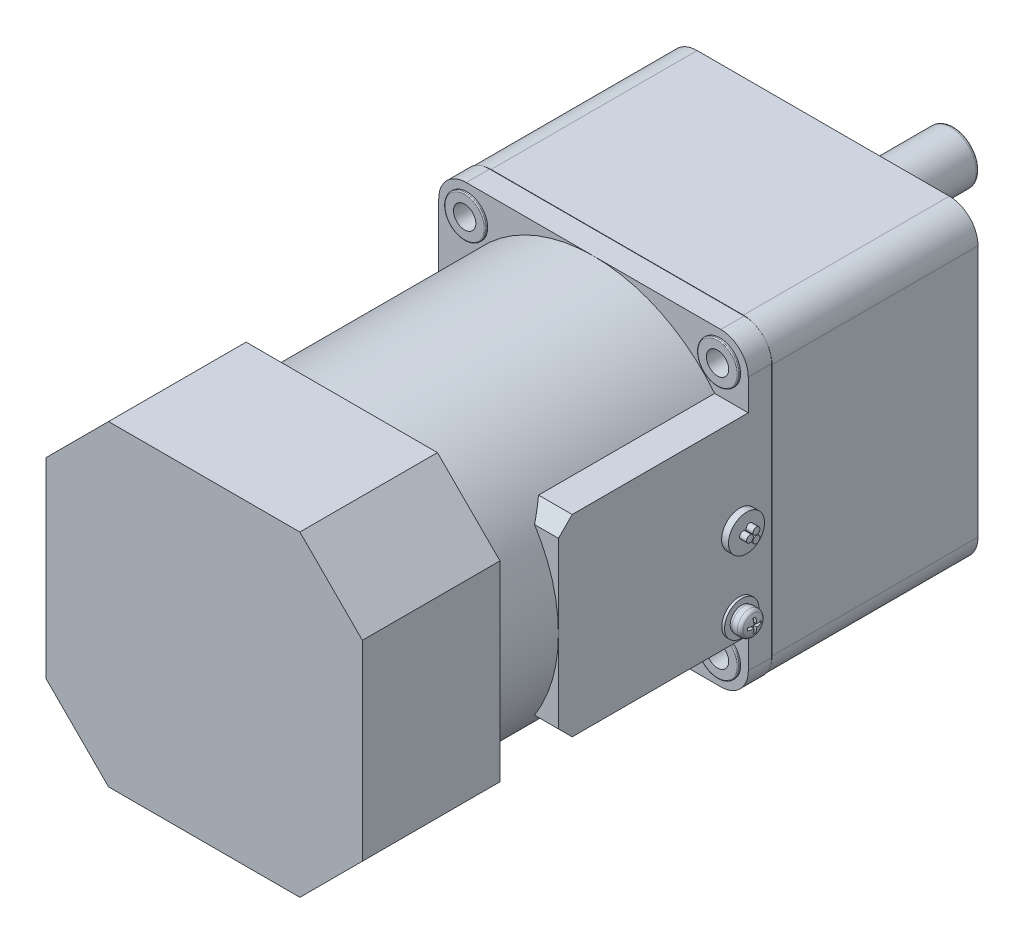
from build123d import *

# Parameters (mm, degrees)
EXTRUDE_1_DEPTH             = 60
EXTRUDE_2_DEPTH             = 6.8
SKETCH_4_W                  = 90
SKETCH_4_H                  = 90
CUT_EXTRUDE_1_DEPTH         = 0.1
EXTRUDE_3_DEPTH             = 45
PATTERN_LINEAR_1_COUNT      = 2
PATTERN_LINEAR_1_PITCH      = 73.539105243
PATTERN_LINEAR_1_COUNT_DIR2 = 2
PATTERN_LINEAR_1_PITCH_DIR2 = 73.539105243
SKETCH_9_W                  = 2
SKETCH_9_H                  = 5.25
SKETCH_10_R                 = 1
EXTRUDE_4_DEPTH             = 2
SKETCH_11_R                 = 1
EXTRUDE_5_DEPTH             = 2
SKETCH_12_R                 = 1
EXTRUDE_6_DEPTH             = 2
CUT_EXTRUDE_2_DEPTH         = 1
EXTRUDE_7_DEPTH             = 40
SKETCH_16_W                 = 67.5
SKETCH_16_H                 = 3.25
PATTERN_LINEAR_2_COUNT      = 2
PATTERN_LINEAR_2_PITCH      = 73.539105243
PATTERN_LINEAR_2_COUNT_DIR2 = 2
PATTERN_LINEAR_2_PITCH_DIR2 = 73.539105243


with BuildPart() as part:
    # 草图1 → 凸台-拉伸1 (new body)
    with BuildSketch(Plane.XY):
        with BuildLine():
            Line((-45, 36.67), (-45, -36.67))
            ThreePointArc((-45, -36.67), (-42.560199487, -42.560199487), (-36.67, -45))
            Line((-36.67, -45), (36.67, -45))
            ThreePointArc((36.67, -45), (42.560199487, -42.560199487), (45, -36.67))
            Line((45, -36.67), (45, 36.67))
            ThreePointArc((45, 36.67), (42.560199487, 42.560199487), (36.67, 45))
            Line((36.67, 45), (-36.67, 45))
            ThreePointArc((-36.67, 45), (-42.560199487, 42.560199487), (-45, 36.67))
        make_face()
    extrude(amount=EXTRUDE_1_DEPTH)

    # 草图2 → 旋转1 (revolve)
    with BuildSketch(Plane(origin=(0, 0, 0), x_dir=(0, 0, -1), z_dir=(1, 0, 0)), mode=Mode.PRIVATE) as revolve_1_sk:
        with BuildLine():
            Line((0, 18), (0, 35))
            Line((0, 35), (6, 35))
            ThreePointArc((6, 35), (6.707106781, 34.707106781), (7, 34))
            Line((7, 34), (7, 25.5))
            Line((7, 25.5), (37, 25.5))
            ThreePointArc((37, 25.5), (37.707106781, 25.207106781), (38, 24.5))
            Line((38, 24.5), (38, 18))
            Line((38, 18), (0, 18))
        make_face()
    revolve(revolve_1_sk.sketch.rotate(Axis((0, 18, -38), (0, 0, 1)), 270), axis=Axis((0, 18, -38), (0, 0, 1)))

    # 草图3 → 凸台-拉伸2 (add)
    with BuildSketch(Plane.XY.offset(60)):
        with BuildLine():
            Line((-45, 37), (-45, -37))
            ThreePointArc((-45, -37), (-42.656854249, -42.656854249), (-37, -45))
            Line((-37, -45), (37, -45))
            ThreePointArc((37, -45), (42.656854249, -42.656854249), (45, -37))
            Line((45, -37), (45, 37))
            ThreePointArc((45, 37), (42.656854249, 42.656854249), (37, 45))
            Line((37, 45), (-37, 45))
            ThreePointArc((-37, 45), (-42.656854249, 42.656854249), (-45, 37))
        make_face()
    extrude(amount=EXTRUDE_2_DEPTH)

    # 草图4 → 切除-拉伸1 (cut)
    with BuildSketch(Plane.XY.offset(60)):
        Rectangle(SKETCH_4_W, SKETCH_4_H)
        with BuildLine():
            Line((-44, 37), (-44, -37))
            ThreePointArc((-44, -37), (-41.949747468, -41.949747468), (-37, -44))
            Line((-37, -44), (37, -44))
            ThreePointArc((37, -44), (41.949747468, -41.949747468), (44, -37))
            Line((44, -37), (44, 37))
            ThreePointArc((44, 37), (41.949747468, 41.949747468), (37, 44))
            Line((37, 44), (-37, 44))
            ThreePointArc((-37, 44), (-41.949747468, 41.949747468), (-44, 37))
        make_face(mode=Mode.SUBTRACT)
    extrude(amount=-CUT_EXTRUDE_1_DEPTH, mode=Mode.SUBTRACT)

    # 草图5 → 旋转2 (revolve)
    with BuildSketch(Plane(origin=(0, 0, 0), x_dir=(0, 0, -1), z_dir=(1, 0, 0)), mode=Mode.PRIVATE) as revolve_2_sk:
        Polygon((-175.5, 0), (-175.5, 26.1), (-180, 26.1), (-180, 42.5), (-179, 43.5), (-175.5, 43.5), (-175.5, 45), (-66.8, 45), (-66.8, 0), align=None)
    revolve(revolve_2_sk.sketch.rotate(Axis((0, 0, 66.8), (0, 0, 1)), 270), axis=Axis((0, 0, 66.8), (0, 0, 1)))

    # 草图6 → 凸台-拉伸3 (add)
    with BuildSketch(Plane(origin=(45, 0, 0), x_dir=(0, 0, -1), z_dir=(1, 0, 0))):
        Polygon((-122, -24), (-118, -28), (-60, -28), (-60, 28), (-118, 28), (-122, 24), align=None)
    extrude(amount=-EXTRUDE_3_DEPTH)

    # 草图7 → 旋转3 (revolve)
    with BuildSketch(Plane(origin=(0, 0, 0), x_dir=(0, 0, -1), z_dir=(0.7071067811865476, 0.7071067811865475, 0)), mode=Mode.PRIVATE) as revolve_3_sk:
        with BuildLine():
            Line((-67.5, -52), (-67.5, -46.3))
            ThreePointArc((-67.5, -46.3), (-67.412132034, -46.087867966), (-67.2, -46))
            Line((-67.2, -46), (-66.8, -46))
            Line((-66.8, -46), (-66.8, -52))
            Line((-66.8, -52), (-67.5, -52))
        make_face()
    revolve_3 = revolve(revolve_3_sk.sketch.rotate(Axis((36.769552622, -36.769552622, 66.8), (0, 0, 1)), 225), axis=Axis((36.769552622, -36.769552622, 66.8), (0, 0, 1)))

    # 阵列(线性)1: Revolve 3 2 × 2
    with Locations(*[(-j * PATTERN_LINEAR_1_PITCH_DIR2, i * PATTERN_LINEAR_1_PITCH, 0) for i in range(PATTERN_LINEAR_1_COUNT) for j in range(PATTERN_LINEAR_1_COUNT_DIR2) if (i, j) != (0, 0)]):
        add(revolve_3)

    # 草图9 → 旋转4 (revolve)
    with BuildSketch(Plane(origin=(0, 0, 0), x_dir=(1, 0, 0), z_dir=(0, 1, 0)), mode=Mode.PRIVATE) as revolve_4_sk:
        with Locations((46, -71.925)):
            Rectangle(SKETCH_9_W, SKETCH_9_H)
    revolve(revolve_4_sk.sketch.rotate(Axis((45, 0, 69.3), (1, 0, 0)), 180), axis=Axis((45, 0, 69.3), (1, 0, 0)))

    # 草图10 → 凸台-拉伸4 (add)
    with BuildSketch(Plane(origin=(47, 0, 0), x_dir=(0, 0, -1), z_dir=(1, 0, 0))):
        with Locations(Location((-70.3, 0, 0), (0, 0, 180))):
            Circle(SKETCH_10_R)
    extrude(amount=EXTRUDE_4_DEPTH)

    # 草图11 → 凸台-拉伸5 (add)
    with BuildSketch(Plane(origin=(47, 0, 0), x_dir=(0, 0, -1), z_dir=(1, 0, 0))):
        with Locations(Location((-68.425, -1.082531755, 0), (0, 0, 180))):
            Circle(SKETCH_11_R)
    extrude(amount=EXTRUDE_5_DEPTH)

    # 草图12 → 凸台-拉伸6 (add)
    with BuildSketch(Plane(origin=(47, 0, 0), x_dir=(0, 0, -1), z_dir=(1, 0, 0))):
        with Locations(Location((-68.425, 1.082531755, 0), (0, 0, 180))):
            Circle(SKETCH_12_R)
    extrude(amount=EXTRUDE_6_DEPTH)

    # 草图13 → 旋转5 (revolve)
    with BuildSketch(Plane(origin=(0, -22, 0), x_dir=(1, 0, 0), z_dir=(0, 1, 0)), mode=Mode.PRIVATE) as revolve_5_sk:
        with BuildLine():
            Line((48.013074887, -73), (46.5, -73))
            Line((46.5, -73), (46.5, -72.85))
            Line((46.5, -72.85), (45.8, -72.85))
            Line((45.8, -72.85), (45.8, -74.5))
            Line((45.8, -74.5), (45, -74.5))
            Line((45, -74.5), (45, -69.5))
            Line((45, -69.5), (49.8, -69.5))
            ThreePointArc((49.8, -69.5), (49.613693389, -70.98356637), (49.066343608, -72.375))
            ThreePointArc((49.066343608, -72.375), (48.625447322, -72.831988372), (48.013074887, -73))
        make_face()
    revolve(revolve_5_sk.sketch.rotate(Axis((45, -22, 69.5), (1, 0, 0)), 180), axis=Axis((45, -22, 69.5), (1, 0, 0)))

    # 草图14 → 切除-拉伸2 (cut)
    with BuildSketch(Plane(origin=(49.8, 0, 0), x_dir=(0, 0, -1), z_dir=(1, 0, 0))):
        Polygon((-71.5, -21.6), (-71.5, -22.4), (-69.9, -22.4), (-69.9, -24), (-69.1, -24), (-69.1, -22.4), (-67.5, -22.4), (-67.5, -21.6), (-69.1, -21.6), (-69.1, -20), (-69.9, -20), (-69.9, -21.6), align=None)
    extrude(amount=-CUT_EXTRUDE_2_DEPTH, mode=Mode.SUBTRACT)

    # 草图15 → 凸台-拉伸7 (add)
    with BuildSketch(Plane.XY.offset(180)):
        Polygon((-46, -27.82), (-27.82, -46), (27.82, -46), (46, -27.82), (46, 27.82), (27.82, 46), (-27.82, 46), (-46, 27.82), align=None)
    extrude(amount=-EXTRUDE_7_DEPTH)

    # 草图16 → 切除-旋转1 (revolve, cut)
    with BuildSketch(Plane(origin=(0, 0, 0), x_dir=(0, 0, -1), z_dir=(0.7071067811865476, 0.7071067811865475, 0)), mode=Mode.PRIVATE) as cut_revolve_1_sk:
        with Locations((-33.75, -50.375)):
            Rectangle(SKETCH_16_W, SKETCH_16_H)
    cut_revolve_1 = revolve(cut_revolve_1_sk.sketch.rotate(Axis((36.769552622, -36.769552622, 0), (0, 0, 1)), 225), axis=Axis((36.769552622, -36.769552622, 0), (0, 0, 1)), mode=Mode.SUBTRACT)

    # 阵列(线性)2: Cut-Revolve 1 2 × 2
    with Locations(*[(-j * PATTERN_LINEAR_2_PITCH_DIR2, i * PATTERN_LINEAR_2_PITCH, 0) for i in range(PATTERN_LINEAR_2_COUNT) for j in range(PATTERN_LINEAR_2_COUNT_DIR2) if (i, j) != (0, 0)]):
        add(cut_revolve_1, mode=Mode.SUBTRACT)


solid = part.part
